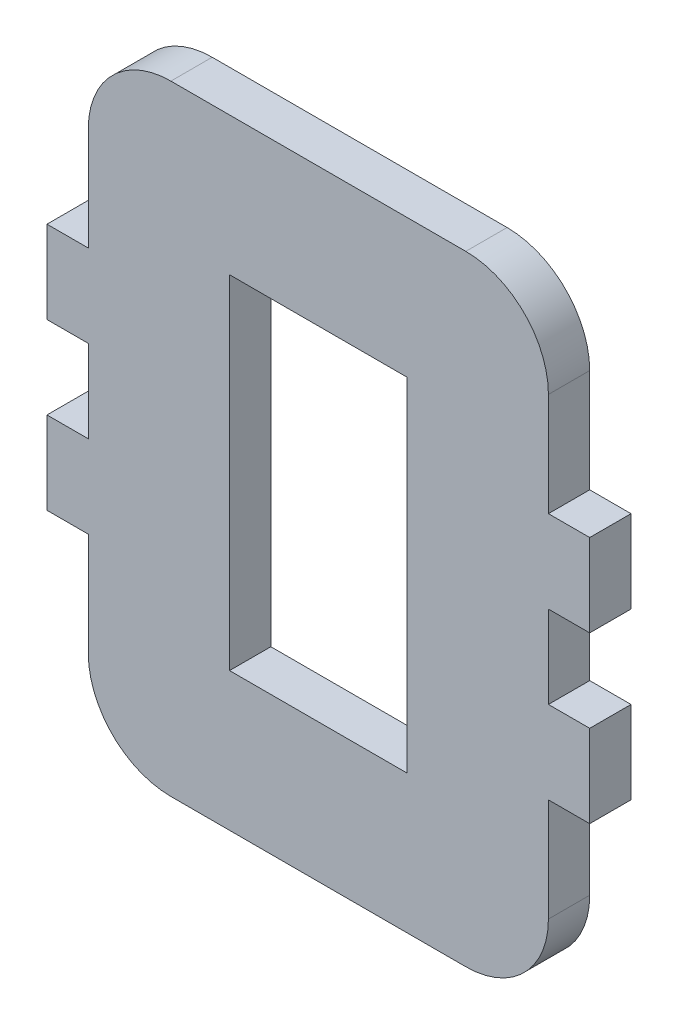
from build123d import *

# Parameters (mm, degrees)
EXTRUDE_1_DEPTH     = 5
SKETCH_2_W          = 21.5
SKETCH_2_H          = 41.5
CUT_EXTRUDE_1_DEPTH = 5
FILLET_1_R          = 10


with BuildPart() as part:
    # 草图1 → 凸台-拉伸1 (new body)
    with BuildSketch(Plane.XY):
        Polygon((-27.85, 37.5), (-27.85, 15), (-32.85, 15), (-32.85, 5), (-27.85, 5), (-27.85, -5), (-32.85, -5), (-32.85, -15), (-27.85, -15), (-27.85, -37.5), (27.85, -37.5), (27.85, -15), (32.85, -15), (32.85, -5), (27.85, -5), (27.85, 5), (32.85, 5), (32.85, 15), (27.85, 15), (27.85, 37.5), align=None)
    extrude(amount=EXTRUDE_1_DEPTH)

    # 草图2 → 切除-拉伸1 (cut)
    with BuildSketch(Plane.XY.offset(5)):
        Rectangle(SKETCH_2_W, SKETCH_2_H)
    extrude(amount=-CUT_EXTRUDE_1_DEPTH, mode=Mode.SUBTRACT)

    # 圆角1
    fillet_1_edges = [part.edges().sort_by_distance(p)[0] for p in [
        (27.85, -37.5, 2.5),
        (-27.85, -37.5, 2.5),
        (-27.85, 37.5, 2.5),
        (27.85, 37.5, 2.5),
    ]]
    fillet(fillet_1_edges, radius=FILLET_1_R)


solid = part.part
